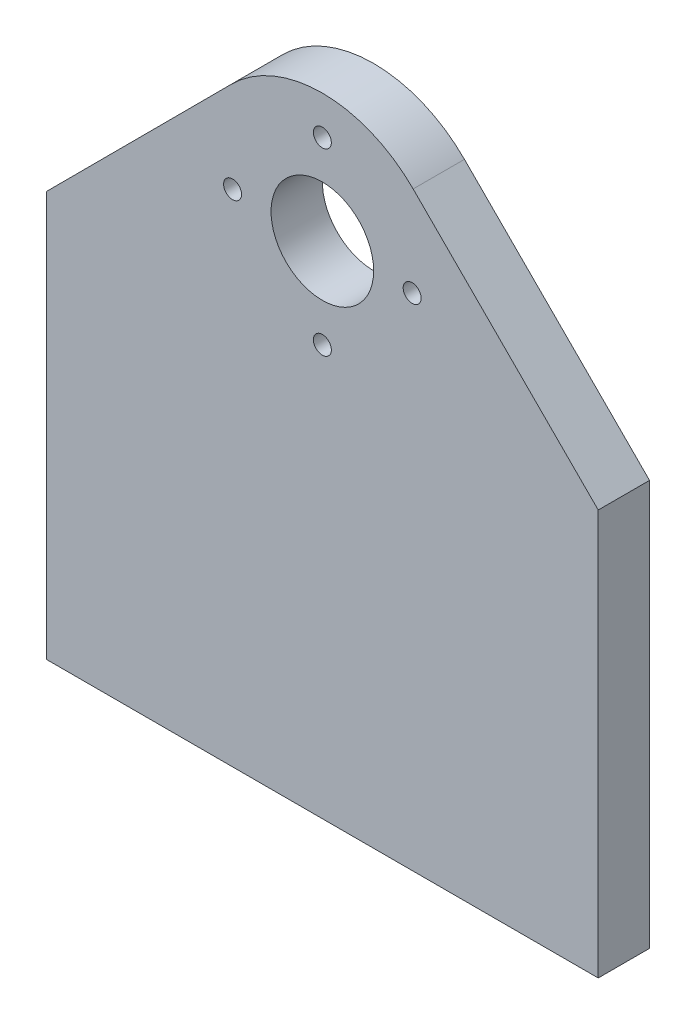
from build123d import *

# Parameters (mm, degrees)
SKETCH1_R           = 40
BOSS_EXTRUDE1_DEPTH = 40
M16_TAPPED_HOLE1_D  = 14


with BuildPart() as part:
    # Sketch1 → Boss-Extrude1 (new body)
    with BuildSketch(Plane.XY):
        with BuildLine():
            Line((0, 0), (430.2, 0))
            Line((430.2, 0), (430.2, 316))
            Line((430.2, 316), (285.889255941, 460.632012878))
            ThreePointArc((285.889255941, 460.632012878), (215.1, 490), (144.310744059, 460.632012878))
            Line((144.310744059, 460.632012878), (0, 316))
            Line((0, 316), (0, 0))
        make_face()
        with Locations((215.1, 390)):
            Circle(SKETCH1_R, mode=Mode.SUBTRACT)
    extrude(amount=BOSS_EXTRUDE1_DEPTH)

    # M16 Tapped Hole1 (through all)
    with Locations(Plane.XY.offset(40)):
        with Locations((215.1, 460), (285.1, 390), (215.1, 320), (145.1, 390)):
            Hole(M16_TAPPED_HOLE1_D / 2)


solid = part.part
